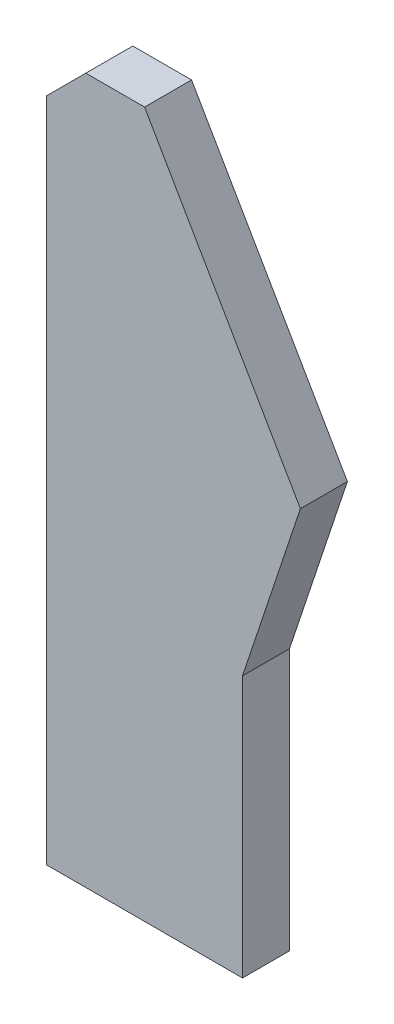
from build123d import *

# Parameters (mm, degrees)
BOSS_EXTRUDE1_DEPTH = 6
CHAMFER1_SIZE       = 10


with BuildPart() as part:
    # Sketch1 → Boss-Extrude1 (new, symmetric)
    with BuildSketch(Plane.XY):
        Polygon((0, 0), (0, 180), (25, 180), (64.770332896, 111.11576279), (50, 66.792003178), (50, 0), align=None)
    extrude(amount=BOSS_EXTRUDE1_DEPTH, both=True)

    # Chamfer1
    chamfer1_edges = [part.edges().sort_by_distance(p)[0] for p in [
        (0, 180, 0),
    ]]
    chamfer(chamfer1_edges, length=CHAMFER1_SIZE)


solid = part.part
